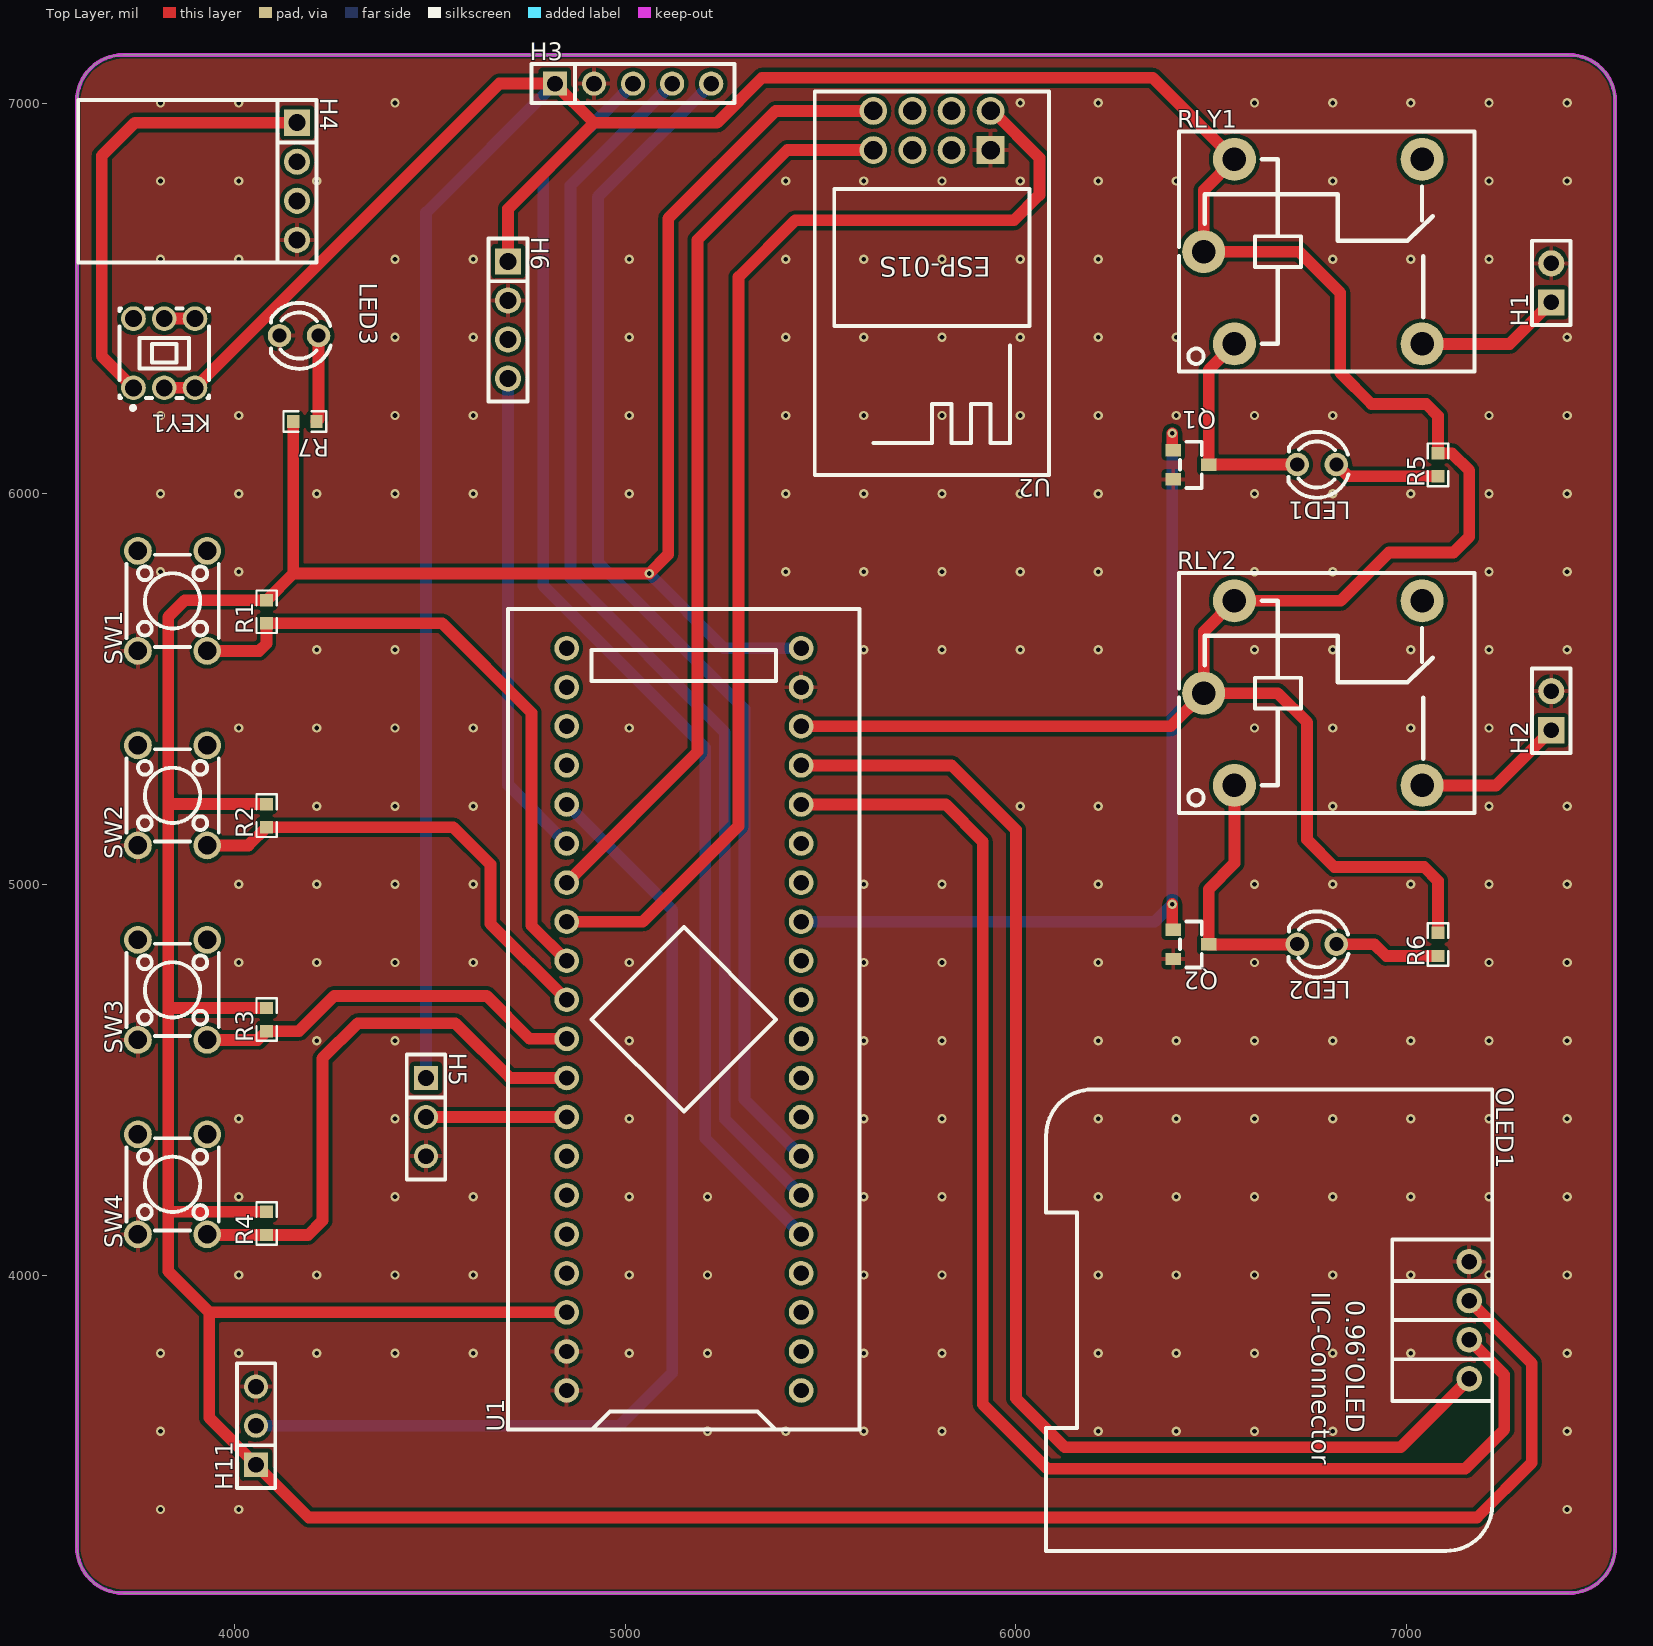
[diagram p0: Top Layer view]
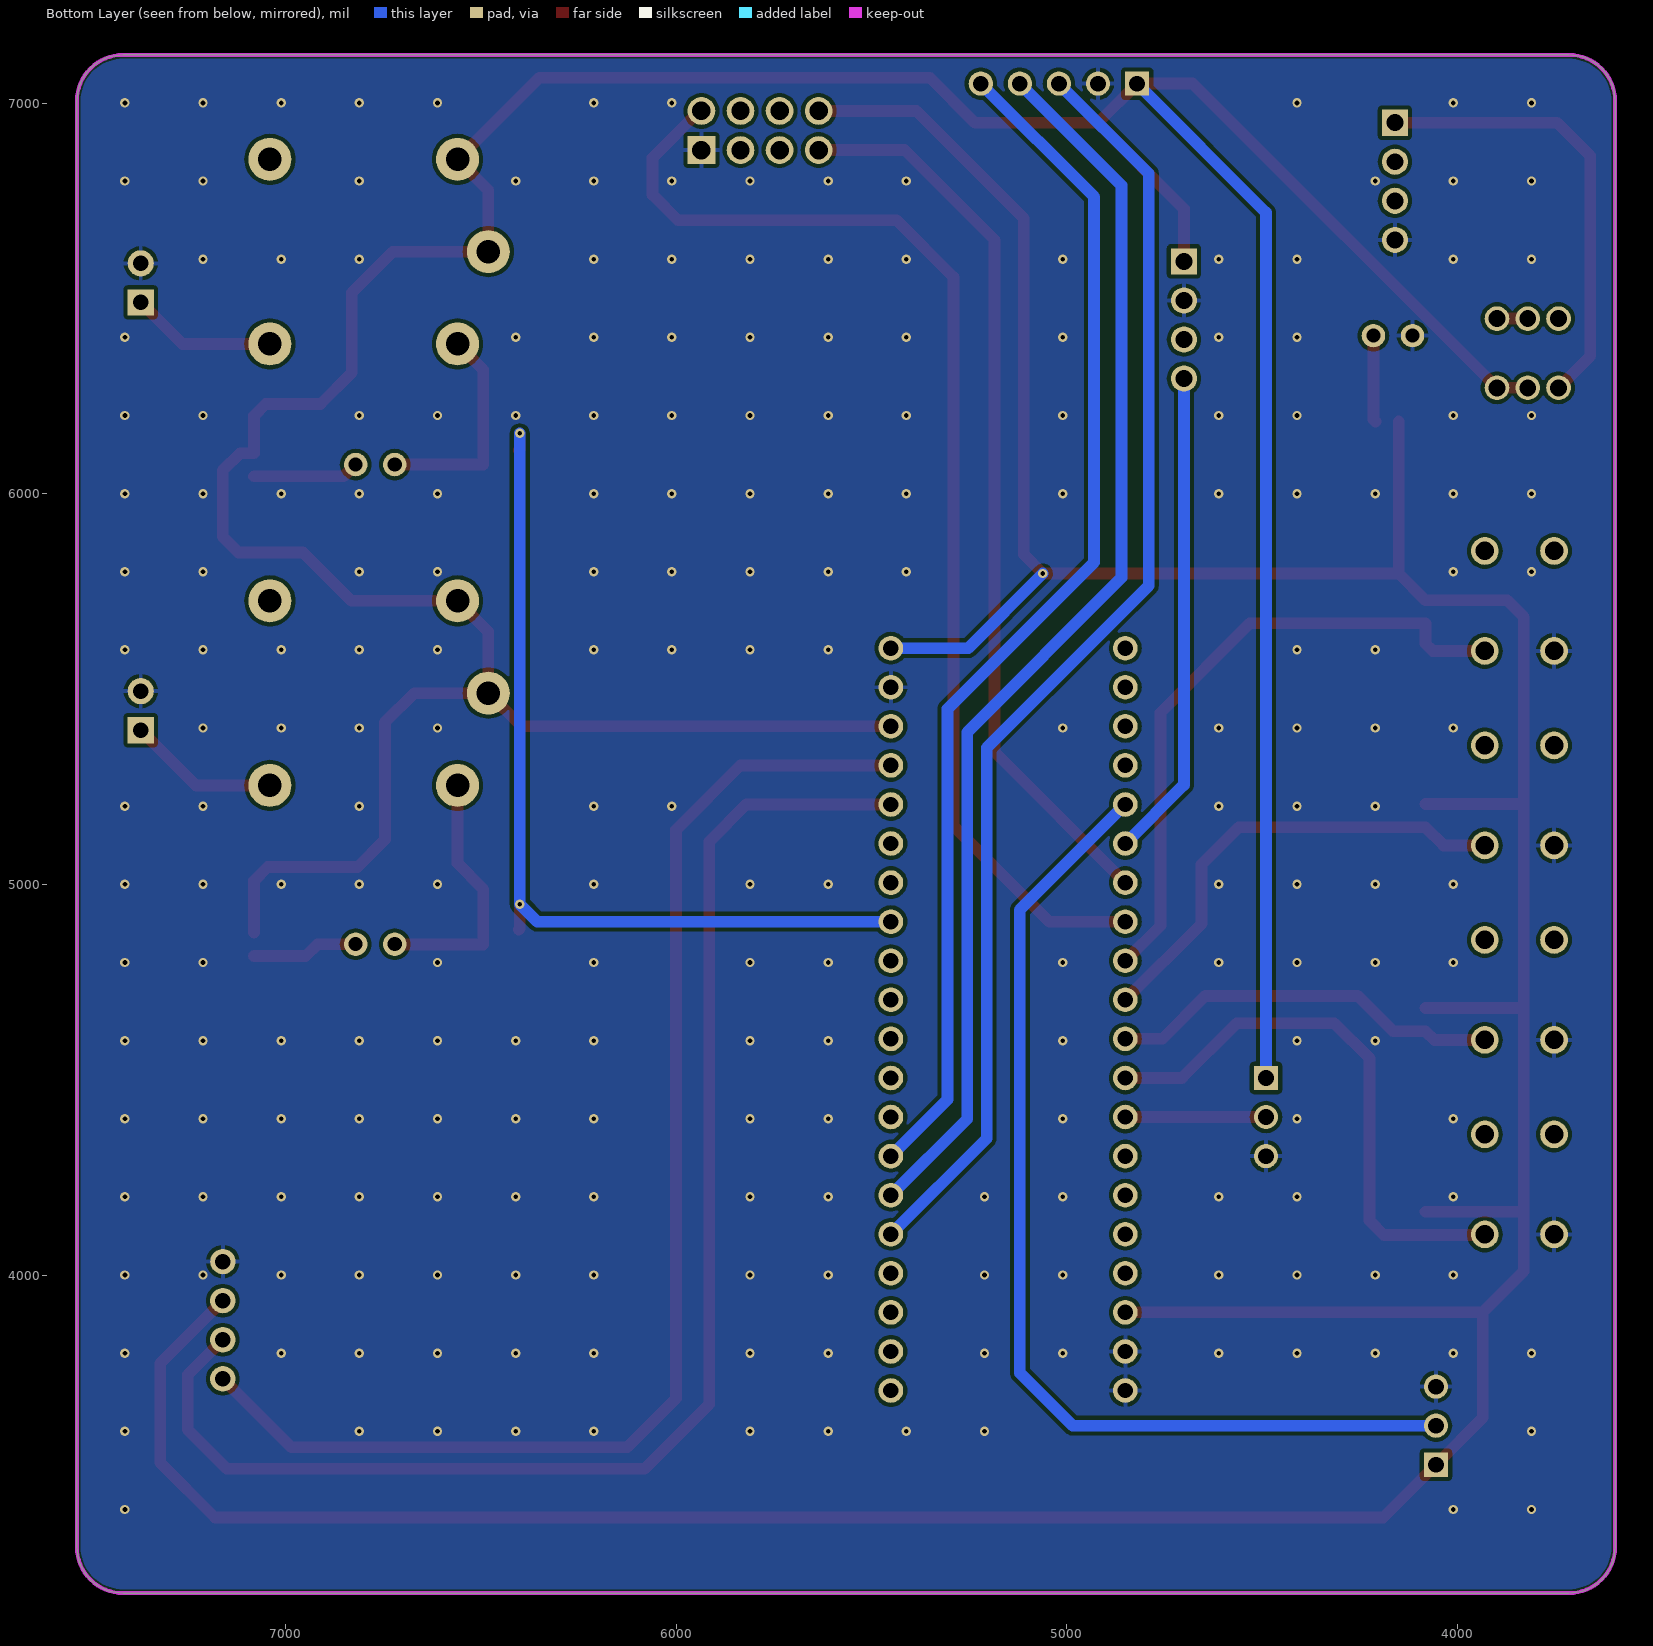
[diagram p1: Bottom Layer view, seen from below]
# Altium PCB MISC49853.pcbdoc
Units mil, origin at the board's own origin, x right, y up, seen from the top; angles counter-clockwise.
Board outline 3937.01 x 3937.01 mil, 2 copper layers (Top Layer, Bottom Layer), stack 62.206 mil thick; 29 components, 46 nets, 133 pads, 222 vias.

## Layer stack, top to bottom
Top Solder Mask Layer: solder mask 0.394, Dk 3.3
Top Layer: signal copper 1.379
Dielectric1: surface 59.449, FR4, Dk 4.5
Bottom Layer: signal copper 1.378
Bottom Solder Mask Layer: solder mask 0.394, Dk 3.3

## Board outline
3714.61,7123.5 ccw(c3714.61,7005.39) 3596.5,7005.39 3596.5,3304.61 ccw(c3714.61,3304.61) 3714.61,3186.5 7415.39,3186.5 ccw(c7415.39,3304.61) 7533.5,3304.61 7533.5,7005.39 ccw(c7415.39,7005.39) 7415.39,7123.5 3714.61,7123.5

## Design rules (kind name [scope] priority, off if disabled: settings)
BoardOutlineClearance copperThickness2oz_1 [All] p2 off: genericclearance=7.99 ignorepadtopadclearanceinfootprint=FALSE except(0: Arc-SplitContinuation Track-SplitContinuation SMDPad-SplitContinuation THPad-SplitContinuation Via-SplitContinuation Fill-SplitContinuation Region-SplitContinuation Poly-SplitContinuation Text-SplitContinuation Hole-SplitContinuation; 5.98: Arc-CutoutEdge Track-CutoutEdge SMDPad-CutoutEdge THPad-CutoutEdge Via-CutoutEdge Text-CutoutEdge; 6.9: Hole-OutlineEdge Hole-CutoutEdge; 10: Poly-OutlineEdge Poly-CutoutEdge; 11.81: Arc-OutlineEdge Track-OutlineEdge SMDPad-OutlineEdge THPad-OutlineEdge Via-OutlineEdge Fill-OutlineEdge Region-OutlineEdge Text-OutlineEdge Fill-CutoutEdge Region-CutoutEdge)
BoardOutlineClearance Plane_innerPlane_1 [All] p4 off: genericclearance=4.02 ignorepadtopadclearanceinfootprint=FALSE except(0: Arc-SplitContinuation Track-SplitContinuation SMDPad-SplitContinuation THPad-SplitContinuation Via-SplitContinuation Fill-SplitContinuation Region-SplitContinuation Poly-SplitContinuation Text-SplitContinuation Hole-SplitContinuation; 5.98: Arc-CutoutEdge Track-CutoutEdge SMDPad-CutoutEdge THPad-CutoutEdge Via-CutoutEdge Text-CutoutEdge; 6.9: Hole-OutlineEdge Hole-CutoutEdge; 10: Poly-OutlineEdge Poly-CutoutEdge; 11.81: Arc-OutlineEdge Track-OutlineEdge SMDPad-OutlineEdge THPad-OutlineEdge Via-OutlineEdge Fill-OutlineEdge Region-OutlineEdge Text-OutlineEdge Fill-CutoutEdge Region-CutoutEdge)
BoardOutlineClearance Copper_copperRegion_1 [All] p6 off: genericclearance=4.02 ignorepadtopadclearanceinfootprint=FALSE except(0: Arc-SplitContinuation Track-SplitContinuation SMDPad-SplitContinuation THPad-SplitContinuation Via-SplitContinuation Fill-SplitContinuation Region-SplitContinuation Poly-SplitContinuation Text-SplitContinuation Hole-SplitContinuation; 5.98: Arc-CutoutEdge Track-CutoutEdge SMDPad-CutoutEdge THPad-CutoutEdge Via-CutoutEdge Text-CutoutEdge; 6.9: Hole-OutlineEdge Hole-CutoutEdge; 10: Poly-OutlineEdge Poly-CutoutEdge; 11.81: Arc-OutlineEdge Track-OutlineEdge SMDPad-OutlineEdge THPad-OutlineEdge Via-OutlineEdge Fill-OutlineEdge Region-OutlineEdge Text-OutlineEdge Fill-CutoutEdge Region-CutoutEdge)
BoardOutlineClearance copperThickness1oz_1 [All] p8: genericclearance=4.02 ignorepadtopadclearanceinfootprint=FALSE except(0: Arc-SplitContinuation Track-SplitContinuation SMDPad-SplitContinuation THPad-SplitContinuation Via-SplitContinuation Fill-SplitContinuation Region-SplitContinuation Poly-SplitContinuation Text-SplitContinuation Hole-SplitContinuation; 5.98: Arc-CutoutEdge Track-CutoutEdge SMDPad-CutoutEdge THPad-CutoutEdge Via-CutoutEdge Text-CutoutEdge; 6.9: Hole-OutlineEdge Hole-CutoutEdge; 10: Poly-OutlineEdge Poly-CutoutEdge; 11.81: Arc-OutlineEdge Track-OutlineEdge SMDPad-OutlineEdge THPad-OutlineEdge Via-OutlineEdge Fill-OutlineEdge Region-OutlineEdge Text-OutlineEdge Fill-CutoutEdge Region-CutoutEdge)
Clearance copperThickness2oz [All] p1 off: gap=7.99 ignorepadtopadclearanceinfootprint=FALSE except(5.98: SMDPad-Track SMDPad-SMDPad THPad-Track SMDPad-THPad THPad-THPad Track-Via SMDPad-Via THPad-Via Via-Via Fill-SMDPad Region-SMDPad Fill-THPad Region-THPad Fill-Via Region-Via Fill-Fill Fill-Region Region-Region Arc-Track Arc-SMDPad Arc-THPad Arc-Via Fill-Arc Region-Arc Arc-Arc Text-Track SMDPad-Text Text-THPad Text-Via Fill-Text Region-Text Arc-Text Text-Text; 6.9: Hole-Track Hole-SMDPad Hole-THPad Hole-Via Fill-Hole Region-Hole Hole-Arc Hole-Text; 10: Poly-Track Poly-SMDPad Poly-THPad Poly-Via Poly-Fill Poly-Region Poly-Poly Poly-Arc Poly-Text Poly-Hole; 11.81: Fill-Track Region-Track)
Clearance Plane_innerPlane [All] p3 off: gap=4.02 ignorepadtopadclearanceinfootprint=FALSE except(5.98: SMDPad-Track SMDPad-SMDPad THPad-Track SMDPad-THPad THPad-THPad Track-Via SMDPad-Via THPad-Via Via-Via Fill-SMDPad Region-SMDPad Fill-THPad Region-THPad Fill-Via Region-Via Fill-Fill Fill-Region Region-Region Arc-Track Arc-SMDPad Arc-THPad Arc-Via Fill-Arc Region-Arc Arc-Arc Text-Track SMDPad-Text Text-THPad Text-Via Fill-Text Region-Text Arc-Text Text-Text; 6.9: Hole-Track Hole-SMDPad Hole-THPad Hole-Via Fill-Hole Region-Hole Hole-Arc Hole-Text; 10: Poly-Track Poly-SMDPad Poly-THPad Poly-Via Poly-Fill Poly-Region Poly-Poly Poly-Arc Poly-Text Poly-Hole; 11.81: Fill-Track Region-Track)
Clearance Copper_copperRegion [All] p5 off: gap=4.02 ignorepadtopadclearanceinfootprint=FALSE except(5.98: SMDPad-Track SMDPad-SMDPad THPad-Track SMDPad-THPad THPad-THPad Track-Via SMDPad-Via THPad-Via Via-Via Fill-SMDPad Region-SMDPad Fill-THPad Region-THPad Fill-Via Region-Via Fill-Fill Fill-Region Region-Region Arc-Track Arc-SMDPad Arc-THPad Arc-Via Fill-Arc Region-Arc Arc-Arc Text-Track SMDPad-Text Text-THPad Text-Via Fill-Text Region-Text Arc-Text Text-Text; 6.9: Hole-Track Hole-SMDPad Hole-THPad Hole-Via Fill-Hole Region-Hole Hole-Arc Hole-Text; 10: Poly-Track Poly-SMDPad Poly-THPad Poly-Via Poly-Fill Poly-Region Poly-Poly Poly-Arc Poly-Text Poly-Hole; 11.81: Fill-Track Region-Track)
Clearance copperThickness1oz [All] p7: gap=4.02 ignorepadtopadclearanceinfootprint=FALSE except(5.98: SMDPad-Track SMDPad-SMDPad THPad-Track SMDPad-THPad THPad-THPad Track-Via SMDPad-Via THPad-Via Via-Via Fill-SMDPad Region-SMDPad Fill-THPad Region-THPad Fill-Via Region-Via Fill-Fill Fill-Region Region-Region Arc-Track Arc-SMDPad Arc-THPad Arc-Via Fill-Arc Region-Arc Arc-Arc Text-Track SMDPad-Text Text-THPad Text-Via Fill-Text Region-Text Arc-Text Text-Text; 6.9: Hole-Track Hole-SMDPad Hole-THPad Hole-Via Fill-Hole Region-Hole Hole-Arc Hole-Text; 10: Poly-Track Poly-SMDPad Poly-THPad Poly-Via Poly-Fill Poly-Region Poly-Poly Poly-Arc Poly-Text Poly-Hole; 11.81: Fill-Track Region-Track)
DiffPairsRouting differentialPair [All] p1: maxlimit=6 minlimit=6 mostfreqgap=6 toplayer_minwidth=5 toplayer_prefwidth=10 toplayer_maxwidth=100 toplayer_mingap=6 toplayer_prefgap=6 toplayer_maxgap=6 bottomlayer_minwidth=5 bottomlayer_prefwidth=10 bottomlayer_maxwidth=100 bottomlayer_mingap=6 bottomlayer_prefgap=6 bottomlayer_maxgap=6 maxuncoupledlength=10
HoleToHoleClearance otherClearance [All] p1: gap=11.81 allowstackedmicrovias=TRUE
Length netLength [All] p1: minlimit=0 maxlimit=0
PasteMaskExpansion pasteMaskExpansion [All] p1: expansion=0
PlaneConnect innerPlane [All] p1: planeconnectstyle=Relief reliefexpansion=20 reliefentries=4 reliefconductorwidth=10 reliefairgap=10
PolygonConnect copperRegion [All] p1: connectstyle=Relief reliefconductorwidth=10 reliefentries=4 polygonreliefangle="90 Angle" airgapwidth=10 via.connectstyle=Relief via.reliefconductorwidth=10 via.reliefentries=4 via.polygonreliefangle="90 Angle" via.airgapwidth=10
RoutingVias viaSize [All] p1: holewidth=12.01 width=24.02 viastyle="Through Hole" minholewidth=11.81 minwidth=19.68 maxholewidth=248.03 maxwidth=393.7
SolderMaskExpansion solderMaskExpansion [IsVia] p1: expansion=-1000 istentingtop=TRUE
SolderMaskExpansion solderMaskExpansion [All] p2: expansion=2 istentingtop=FALSE
Width copperThickness2oz_2 [All] p1 off: maxlimit=100 minlimit=8 preferedwidth=10
Width copperThickness1oz_2 [All] p2: maxlimit=100 minlimit=5 preferedwidth=10

## Components (designator, comment, footprint, x,y, rotation, side; value= is the part's Value field where it differs from the comment)
H1 "" HDR-TH_2P-P2.54-V-F 7370,6540 r90 top
H2 "" HDR-TH_2P-P2.54-V-F 7370,5445 r90 top
H3 "" HDR-TH_5P-P2.54-V-F 5020,7050 r0 top
H4 "" HDR-TH_4P-P2.54-V-F 4160,6800 r270 top
H5 "" HDR-TH_3P-P2.54-V-F 4490,4405 r270 top
H6 "" HDR-TH_4P-P2.54-V-F 4700,6445 r270 top
H11 "" HDR-TH_3P-P2.54-V-F 4055,3615 r90 top
KEY1 "Self-locking switch 5.8Z white-grey-white 260G" SW-TH_6P-L5.8-W5.8-P2.00-LS4.5-TR 3820,6360 r180 top
LED1 "" LED_TH-3mm 6770,6075 r180 top
LED2 "" LED_TH-3mm 6770,4847.46 r180 top
LED3 "" LED_TH-3mm 4165,6405 r180 top
OLED1 "" 0.96OLED_4P 7160,3885 r270 top
Q1 "" S8050_SOT-23 6447.93,6074.41 r180 top
Q2 "" S8050_SOT-23 6447.93,4846.87 r180 top
R1 "10K" R0603 4082.02,5698.23 r90 top
R2 "10K" R0603 4082.02,5176.36 r90 top
R3 "10K" R0603 4082.02,4654.49 r90 top
R4 "10K" R0603 4082.02,4132.62 r90 top
R5 "1K" R0603 7080,6074.41 r90 top
R6 "1K" R0603 7080,4846.87 r90 top
R7 "1K" R0603 4180,6185 r180 top
RLY1 "SRD-05VDC-SL-C" RELAY-TH_SRD-XXVDC-XL-C 6760,6620 r0 top
RLY2 "SRD-05VDC-SL-C" RELAY-TH_SRD-XXVDC-XL-C 6760,5490 r0 top
SW1 "" SW-TH_4P-L6.0-W6.0-P4.50-LS6.5 3841.42,5725.93 r90 top
SW2 "" SW-TH_4P-L6.0-W6.0-P4.50-LS6.5 3841.42,5228.16 r90 top
SW3 "" SW-TH_4P-L6.0-W6.0-P4.50-LS6.5 3841.42,4730.39 r90 top
SW4 "" SW-TH_4P-L6.0-W6.0-P4.50-LS6.5 3841.42,4232.62 r90 top
U1 "STM32F103C8T6-Card" CONN-TH_L53.3-W22.9_STM32F103C8T6-CARD 5150,4655 r90 top
U2 "ESP-01S" WIFIM-TH_ESP-01S 5785,6930 r180 top

## Footprints (in the part's own frame and the unit in brackets; to place one, negate y for a bottom-side part, rotate by r counter-clockwise, add the part's x,y. Pads: shape width x height; smd on the part's side, far side on the other; paste and mask are expansions set on the pad)
0.96OLED_4P [mm]
  round 1.65 hole 1 copper offset 0,0: 1(-3.81,-0.001) 2(-1.27,0.002) 3(1.27,0.002) 4(3.81,0.002)
  silkscreen extent -15,-27.5 15,1.5
CONN-TH_L53.3-W22.9_STM32F103C8T6-CARD [mm]
  round 1.6 hole 1: 1(-24.13,-7.62) 2(-21.59,-7.62) 3(-19.05,-7.62) 4(-16.51,-7.62) 5(-13.97,-7.62) 6(-11.43,-7.62) 7(-8.89,-7.62) 8(-6.35,-7.62) 9(-3.81,-7.62) 10(-1.27,-7.62) 11(1.27,-7.62) 12(3.81,-7.62) 13(6.35,-7.62) 14(8.89,-7.62) 15(11.43,-7.62) 16(13.97,-7.62) 17(16.51,-7.62) 18(19.05,-7.62) 19(21.59,-7.62) 20(24.13,-7.62) 21(24.13,7.62) 22(21.59,7.62) 23(19.05,7.62) 24(16.51,7.62) 25(13.97,7.62) 26(11.43,7.62) 27(8.89,7.62) 28(6.35,7.62) 29(3.81,7.62) 30(1.27,7.62) 31(-1.27,7.62) 32(-3.81,7.62) 33(-6.35,7.62) 34(-8.89,7.62) 35(-11.43,7.62) 36(-13.97,7.62) 37(-16.51,7.62) 38(-19.05,7.62) 39(-21.59,7.62) 40(-24.13,7.62)
  silkscreen extent -26.67,-11.43 26.67,11.43
HDR-TH_2P-P2.54-V-F [mm]
  rect 1.7x1.7 hole 1: 1(-1.27,0)
  round 1.7 hole 1: 2(1.27,0)
  silkscreen extent -2.74,-1.25 2.74,1.25
HDR-TH_3P-P2.54-V-F [mil]
  rect 62x62 hole 40.16: 1(-100,0)
  round 62 hole 40.16: 2(0,0) 3(100,0)
  silkscreen extent -160,-49 160,49
HDR-TH_4P-P2.54-V-F [mm]
  rect 1.7x1.7 hole 1.1: 1(-3.81,0)
  round 1.7 hole 1.1: 2(-1.27,0) 3(1.27,0) 4(3.81,0)
  silkscreen extent -5.29,-1.27 5.29,1.27
HDR-TH_5P-P2.54-V-F [mil]
  rect 62x62 hole 40.16: 1(-200,0)
  round 62 hole 40.16: 2(-100,0) 3(0,0) 4(100,0) 5(200,0)
  silkscreen extent -260,-50 260,50
LED_TH-3mm [mil]
  round 60 hole 36 paste+0 mask+2: 1(-50,0) 2(50,0)
  silkscreen extent -81,-84 72,85
R0603 [mil]
  rect 31.75x34.02 smd paste-3937.01 mask+2: 1(-29.66,0) 2(29.66,0)
  silkscreen extent -55,-26 55,26
RELAY-TH_SRD-XXVDC-XL-C [mil]
  round 110 hole 60: 1(-200.79,-236.22) 2(279.52,-236.2) 3(279.53,236.2) 4(-200.79,236.22) 5(-279.53,0)
  silkscreen extent -342,-307 413,307
S8050_SOT-23 [mm]
  rect 1x0.8 smd paste+0 mask+0.051: 1(1.15,-0.95) 2(1.15,0.95) 3(-1.15,0)
  silkscreen extent -0.7,-1.5 0.7,1.5
SW-TH_4P-L6.0-W6.0-P4.50-LS6.5 [mm]
  round 1.8 hole 1.2: 1(-3.25,2.25) 2(3.25,2.25) 3(-3.25,-2.25) 4(3.25,-2.25)
  silkscreen extent -3,-3 3,3
SW-TH_6P-L5.8-W5.8-P2.00-LS4.5-TR [mm]
  round 1.6 hole 1.1: 1(2,2.25) 2(0,2.25) 3(-2,2.25) 4(-2,-2.25) 5(0,-2.25) 6(2,-2.25)
  silkscreen extent -2.9,-2.9 2.9,3.68
WIFIM-TH_ESP-01S [mm]
  rect 1.8x1.8 hole 1.2: 1(-3.81,1.27)
  round 1.8 hole 1.2: 2(-1.27,1.27) 3(1.27,1.27) 4(3.81,1.27) 5(3.81,-1.27) 6(1.27,-1.27) 7(-1.27,-1.27) 8(-3.81,-1.27)
  silkscreen extent -7.62,-2.54 7.62,22.4

## Via types
v1: diameter 24.02, hole 12, Top Layer to Bottom Layer, 222 vias

## Nets (pads, with @x,y where several pads share a name; then routed paths per layer and width w, separated by ;. In a path a pad name is that pad's centre, name@x,y a point inside that pad or via, vN(x,y) a via of type N, cw(c..) or ccw(c..) an arc to the next point about the centre after c; other vN are vias at no path point)
$1N17124: LED1.2 Q1.3 RLY1.1 | length 563.8
  Top Layer w30: RLY1.1 6493.2,6317.77 Q1.3 6493.8,6075 LED1.2
$1N17127: H1.1 RLY1.2 | length 374.5
  Top Layer w30: RLY1.2 7263.8,6383.8 H1.1
$1N17131: LED1.1 R5.1 | length 272.5
  Top Layer w30: LED1.1 6850.25,6044.75 R5.1
$1N17132: LED2.1 R6.1 | length 272.5
  Top Layer w30: LED2.1 6917.54,4847.46 6947.79,4817.21 R6.1
$1N17136: H2.1 RLY2.2 | length 389
  Top Layer w30: RLY2.2 7228.8,5253.8 H2.1
$1N17139: LED2.2 Q2.3 RLY2.1 | length 661.3
  Top Layer w30: RLY2.1 6559.21,5054.21 6493.2,4988.2 Q2.3 6719.41,4846.87 LED2.2
$1N17146: LED3.1 R7.1 | length 222.2
  Top Layer w30: R7.1 4215,6190.34 LED3.1
$1N17148: KEY1.4 KEY1.5 | length 78.7
  Top Layer w30: KEY1.5 KEY1.4
+5V: H3.1 H5.1 H6.1 KEY1.2 KEY1.3 R5.2 R6.2 RLY1.4 RLY1.5 RLY2.4 RLY2.5 U1.18 | length 11002.4
  Top Layer w30: KEY1.2 KEY1.3 4677.32,7050 H3.1 4920,6950 ; H6.1 4700,6730 4920,6950 ; U1.18 6395.47,5405 RLY2.5 ; R6.2 7080,5010 7045,5045 6815,5045 6745,5115 6745,5415 6670,5490 RLY2.5 ; 4920,6950 5235,6950 5350,7065 6350.43,7065 RLY1.4 6480.47,6777.48 RLY1.5 6725,6620 6830,6515 6830,6310 6910,6230 7050,6230 7080,6200 R5.2 7115.93,6104.07 7160,6060 7160,5890 7120,5850 6955,5850 6831.22,5726.22 RLY2.4 6480.47,5647.48 RLY2.5
  Bottom Layer w30: H5.1 4490,6720 H3.1
GND: H1.2 H2.2 H3.2 H4.4 H5.3 H6.2 H11.3 LED3.2 OLED1.1 Q1.2 Q2.2 SW1.1 SW2.1 SW3.1 SW4.1 U1.19 U1.39 U1.40 U2.1
  other v1: 3810.6,3400.6 4010.6,3400.6 7410.6,3400.6 3810.6,3600.6 5210.6,3600.6 5410.6,3600.6 5610.6,3600.6 5810.6,3600.6 6210.6,3600.6 6410.6,3600.6 6610.6,3600.6 6810.6,3600.6 7410.6,3600.6 3810.6,3800.6 4010.6,3800.6 4210.6,3800.6 4410.6,3800.6 4610.6,3800.6 5010.6,3800.6 5210.6,3800.6 5610.6,3800.6 5810.6,3800.6 6210.6,3800.6 6410.6,3800.6 6610.6,3800.6 6810.6,3800.6 7010.6,3800.6 7410.6,3800.6 4010.6,4000.6 4210.6,4000.6 4410.6,4000.6 4610.6,4000.6 5010.6,4000.6 5210.6,4000.6 5610.6,4000.6 5810.6,4000.6 6210.6,4000.6 6410.6,4000.6 6610.6,4000.6 6810.6,4000.6 7010.6,4000.6 7210.6,4000.6 7410.6,4000.6 4010.6,4200.6 4410.6,4200.6 4610.6,4200.6 5010.6,4200.6 5210.6,4200.6 5610.6,4200.6 5810.6,4200.6 6210.6,4200.6 6410.6,4200.6 6610.6,4200.6 6810.6,4200.6 7010.6,4200.6 7210.6,4200.6 7410.6,4200.6 4010.6,4400.6 4410.6,4400.6 5010.6,4400.6 5610.6,4400.6 5810.6,4400.6 6210.6,4400.6 6410.6,4400.6 6610.6,4400.6 6810.6,4400.6 7010.6,4400.6 7210.6,4400.6 7410.6,4400.6 4210.6,4600.6 4410.6,4600.6 5010.6,4600.6 5610.6,4600.6 5810.6,4600.6 6210.6,4600.6 6410.6,4600.6 6610.6,4600.6 6810.6,4600.6 7010.6,4600.6 7210.6,4600.6 7410.6,4600.6 4010.6,4800.6 4210.6,4800.6 4410.6,4800.6 4610.6,4800.6 5010.6,4800.6 5610.6,4800.6 5810.6,4800.6 6210.6,4800.6 6610.6,4800.6 7210.6,4800.6 7410.6,4800.6 4010.6,5000.6 4210.6,5000.6 4410.6,5000.6 4610.6,5000.6 5610.6,5000.6 5810.6,5000.6 6210.6,5000.6 6610.6,5000.6 6810.6,5000.6 7010.6,5000.6 7210.6,5000.6 7410.6,5000.6 4210.6,5200.6 4410.6,5200.6 4610.6,5200.6 6010.6,5200.6 6210.6,5200.6 6810.6,5200.6 7210.6,5200.6 7410.6,5200.6 4010.6,5400.6 4210.6,5400.6 4410.6,5400.6 4610.6,5400.6 5010.6,5400.6 6610.6,5400.6 6810.6,5400.6 7010.6,5400.6 7210.6,5400.6 4210.6,5600.6 4410.6,5600.6 5610.6,5600.6 5810.6,5600.6 6010.6,5600.6 6210.6,5600.6 6610.6,5600.6 6810.6,5600.6 7010.6,5600.6 7210.6,5600.6 7410.6,5600.6 3810.6,5800.6 4010.6,5800.6 5410.6,5800.6 5610.6,5800.6 5810.6,5800.6 6010.6,5800.6 6210.6,5800.6 6610.6,5800.6 6810.6,5800.6 7210.6,5800.6 7410.6,5800.6 3810.6,6000.6 4010.6,6000.6 4210.6,6000.6 4410.6,6000.6 4610.6,6000.6 5010.6,6000.6 5410.6,6000.6 5610.6,6000.6 5810.6,6000.6 6010.6,6000.6 6210.6,6000.6 6610.6,6000.6 6810.6,6000.6 7010.6,6000.6 7210.6,6000.6 7410.6,6000.6 3810.6,6200.6 4010.6,6200.6 4410.6,6200.6 4610.6,6200.6 5010.6,6200.6 5410.6,6200.6 5610.6,6200.6 5810.6,6200.6 6010.6,6200.6 6210.6,6200.6 6410.6,6200.6 6610.6,6200.6 6810.6,6200.6 7210.6,6200.6 7410.6,6200.6 4410.6,6400.6 4610.6,6400.6 5010.6,6400.6 5410.6,6400.6 5610.6,6400.6 5810.6,6400.6 6010.6,6400.6 6210.6,6400.6 6410.6,6400.6 7410.6,6400.6 3810.6,6600.6 4010.6,6600.6 4410.6,6600.6 4610.6,6600.6 5010.6,6600.6 5410.6,6600.6 5610.6,6600.6 5810.6,6600.6 6010.6,6600.6 6210.6,6600.6 6810.6,6600.6 7010.6,6600.6 7210.6,6600.6 3810.6,6800.6 4010.6,6800.6 4210.6,6800.6 5410.6,6800.6 5610.6,6800.6 5810.6,6800.6 6010.6,6800.6 6210.6,6800.6 6410.6,6800.6 6810.6,6800.6 7210.6,6800.6 7410.6,6800.6 3810.6,7000.6 4010.6,7000.6 4410.6,7000.6 6010.6,7000.6 6210.6,7000.6 6610.6,7000.6 6810.6,7000.6 7010.6,7000.6 7210.6,7000.6 7410.6,7000.6
IN_5V: H4.1 KEY1.1 | length 1162.4
  Top Layer w30: KEY1.1 3660,6352.68 3660,6865 3745,6950 H4.1
NRST: U1.37
PA0: H11.2 U1.25 | length 2687.8
  Bottom Layer w30: H11.2 4985,3615 5120,3750 5120,4935 U1.25
PA1: H6.4 U1.26 | length 1252.1
  Bottom Layer w30: H6.4 4700,5255 U1.26
PA2: U1.27 U2.4 | length 2329
  Top Layer w30: U1.27 5185,5340 5185,6650 5415,6880 U2.4
PA3: U1.28 U2.8 | length 3073.2
  Top Layer w30: U1.28 5045,4905 5290,5150 5290,6555 5435,6700 5995,6700 6060,6765 6060,6860 5940,6980 U2.8
PA4: R1.1 SW1.3 U1.29 | length 1656.4
  Top Layer w30: SW1.3 4062.98,5597.98 4082.02,5617.02 R1.1 4531.43,5668.57 4760,5440 4760,4895 U1.29
PA5: R2.1 SW2.3 U1.30 | length 1211.1
  Top Layer w30: SW2.3 4035.53,5100.21 R2.1 4560,5146.7 4655,5051.7 4655,4900 U1.30
PA6: R3.1 SW3.3 U1.31 | length 1012.2
  Top Layer w30: SW3.3 4059.63,4602.44 R3.1 4164.83,4624.83 4255,4715 4645,4715 4755,4605 U1.31
PA7: R4.1 SW4.3 U1.32 | length 1446.3
  Top Layer w30: SW4.3 3931.71,4102.96 R4.1 4187.96,4102.96 4225,4140 4225,4555 4315,4645 4565,4645 4705,4505 U1.32
PA8: H3.3 U1.5 | length 3313.6
  Bottom Layer w30: H3.3 4790,6820 4790,5765 5205,5350 5205,4350 U1.5
PA9: H3.4 U1.6 | length 3197.1
  Bottom Layer w30: H3.4 4860,6790 4860,5785 5255,5390 5255,4400 U1.6
PA10: H3.5 U1.7 | length 3080.5
  Bottom Layer w30: H3.5 4930,6760 4930,5825 5305,5450 5305,4450 U1.7
PA11: U1.8
PA12: U1.9
PA15: U1.10
PB0: H5.2 U1.33 | length 360
  Top Layer w30: H5.2 U1.33
PB1: U1.34
PB3: U1.11
PB4: U1.12
PB5: Q1.1 Q2.1 U1.13 | length 2284.8
  Top Layer w30: v1(6400,4950) 6400,4886.92 Q2.1 ; v1(6400,6155) 6400,6114.46 Q1.1
  Bottom Layer w30: U1.13 6355,4905 v1(6400,4950) v1(6400,6155)
PB6: U1.14
PB7: U1.15
PB8: OLED1.3 U1.16 | length 3656.4
  Top Layer w30: U1.16 5820,5205 5915,5110 5915,3670 6080,3505 7150,3505 7250,3605 7250,3745.05 OLED1.3@7160.05,3835
PB9: OLED1.4 U1.17 | length 3357.7
  Top Layer w30: U1.17 5835,5305 6000,5140 6000,3685 6125,3560 6985.05,3560 OLED1.4@7160.05,3735
PB10: U1.35
PB11: U1.36
PB12: U1.1
PB13: U1.2
PB14: U1.3
PB15: U1.4
PC13: U1.22
PC14: U1.23
PC15: U1.24
VBAT: U1.21
VCC: H11.1 OLED1.2 R1.2 R2.2 R3.2 R4.2 R7.2 U1.20 U1.38 U2.5 | length 11499.9
  Top Layer w30: R4.2 3831.67,4162.28 3830,4160.6 ; R3.2 3832.05,4684.15 3830,4686.2 ; R2.2 3834.81,5206.02 3830,5210.83 ; R7.2 4150.34,5796.21 ; U1.38 3935,3905 ; U2.5 5385,6980 5110,6705 5110,5845 v1(5061.21,5796.21) 4150.34,5796.21 ; OLED1.2@7160.05,3935 7320,3775.05 7320,3520 7180,3380 4190,3380 H11.1 3935,3635 3935,3905 ; 3830,4160.6 3830,4010 3935,3905 ; 3830,4160.6 3830,4686.2 ; 3830,4686.2 3830,5210.83 ; 3830,5210.83 3830,5685 3872.89,5727.89 R1.2 4150.34,5796.21
  Bottom Layer w30: v1(5061.21,5796.21) 5252.42,5605 U1.20
pads on no net: H4.2 H4.3 H6.3 KEY1.6 RLY1.3 RLY2.3 SW1.2 SW1.4 SW2.2 SW2.4 SW3.2 SW3.4 SW4.2 SW4.4 U2.2 U2.3 U2.6 U2.7

## Polygon pours and split planes (outlines as drawn)
GND on Bottom Layer (solid, remove dead copper, pour order 2): 3525,7245 3525,3080 7700,3080 7700,7245
GND on Top Layer (solid, remove dead copper, pour order 2): 3000,7415 3000,3000 7930,3000 7930,7415

## Keep-outs
Board Outline Layer:
  the board outline again, w10

## Silkscreen, mask and mechanical layers (free items; w line width, h text height)
Top Silkscreen Layer:
  lines w10: 3600,6591.73 3600,7008.27 4210,7008.27 4210,6591.73 3600,6591.73